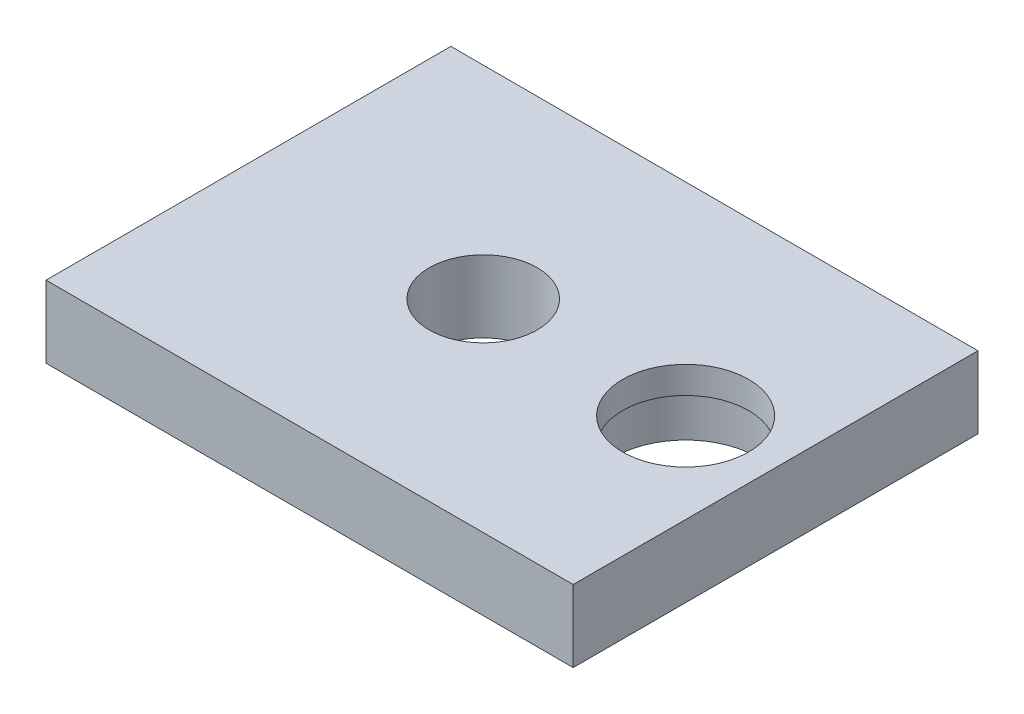
SolidWorks part; units mm, degrees
ref_plane "前视基准面" through (0, 0, 0) normal (0, 0, 1) x (1, 0, 0)
ref_plane "上视基准面" through (0, 0, 0) normal (0, 1, 0) x (1, 0, 0)
ref_plane "右视基准面" through (0, 0, 0) normal (1, 0, 0) x (0, 0, -1)
sketch "草图1" plane through (0, 0, 0) normal (0, 1, 0) x (1, 0, 0)
  line L1 (-146.5, -112.5) -> (146.5, -112.5)
  line L2 (-146.5, -112.5) -> (-146.5, 112.5)
  line L3 (-146.5, 112.5) -> (146.5, 112.5)
  line L4 (146.5, -112.5) -> (146.5, 112.5)
  line L5 (-146.5, -112.5) -> (146.5, 112.5) construction
  line L6 (-146.5, 112.5) -> (146.5, -112.5) construction
  point P0 (0, 0)
  dimension "D1" = 225
  dimension "D2" = 293
extrude "凸台-拉伸1" add sketch "草图1" along normal blind 40
sketch "草图2" plane through (0, 0, 0) normal (0, -1, 0) x (1, 0, 0)
  line L0 (146.5, 112.5) -> (146.5, -112.5) construction
  line L1 (-146.5, 112.5) -> (146.5, 112.5) construction
  circle A0 centre (96.5, 0) radius 40
  dimension "D1" = 80
  dimension "D2" = 50
  dimension "D3" = 112.5
extrude "切除-拉伸1" cut sketch "草图2" against normal blind 25
sketch "草图3" plane through (0, 0, 0) normal (0, -1, 0) x (1, 0, 0)
  line L0 (146.5, 112.5) -> (146.5, -112.5) construction
  line L1 (-146.5, 112.5) -> (146.5, 112.5) construction
  circle A0 centre (-16, 0) radius 30
  dimension "D1" = 60
  dimension "D2" = 162.5
  dimension "D3" = 112.5
extrude "切除-拉伸2" cut sketch "草图3" against normal through all
sketch "草图4" plane through (0, 0, 0) normal (0, -1, 0) x (1, 0, 0)
  line L0 (146.5, 112.5) -> (146.5, -112.5) construction
  circle A0 centre (96.5, 0) radius 35
  dimension "D1" = 70
  dimension "D2" = 50
  dimension "D3" = 112.5
extrude "切除-拉伸3" cut sketch "草图4" against normal through all
